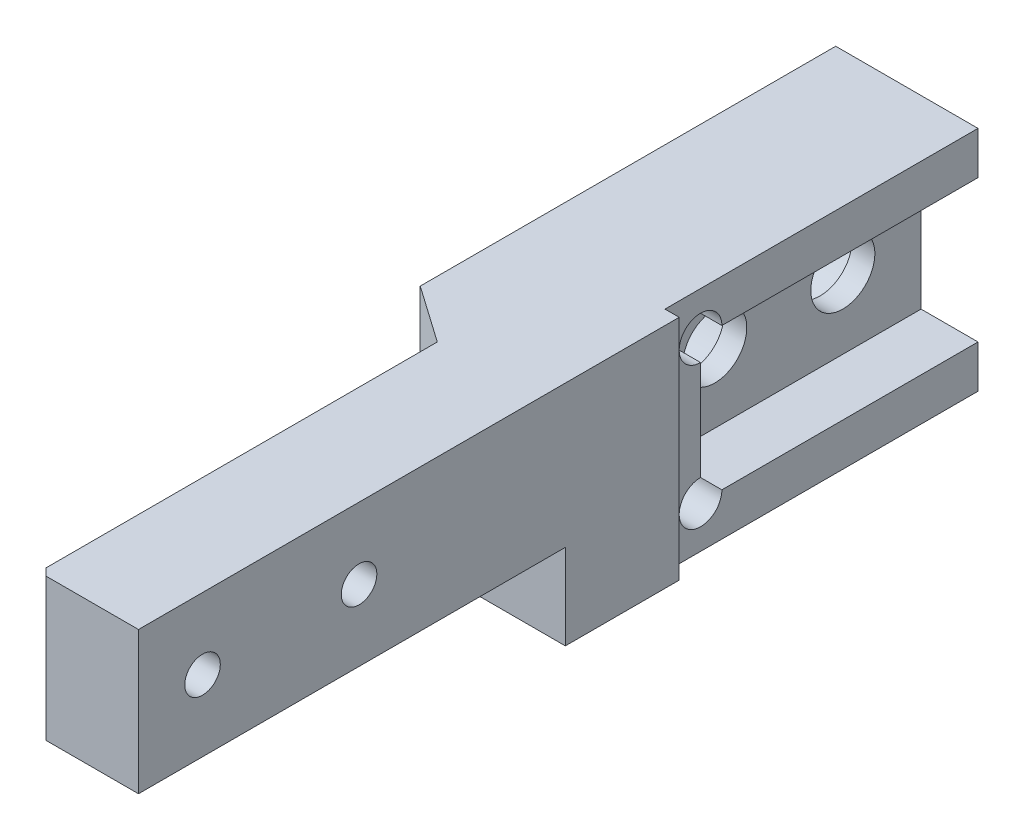
SolidWorks part; units mm, degrees
material "AL6061"
ref_plane "前视基准面" through (0, 0, 0) normal (0, 0, 1) x (1, 0, 0)
ref_plane "上视基准面" through (0, 0, 0) normal (0, 1, 0) x (1, 0, 0)
ref_plane "右视基准面" through (0, 0, 0) normal (1, 0, 0) x (0, 0, -1)
sketch "草图1" plane through (0, 0, 0) normal (0, 1, 0) x (1, 0, 0)
  line L1 (-10, 30) -> (10, 30)
  line L2 (-10, 30) -> (-10, -30)
  line L3 (-10, -30) -> (10, -30)
  line L4 (10, 30) -> (10, -30)
  line L5 (-10, 30) -> (10, -30) construction
  line L6 (-10, -30) -> (10, 30) construction
  point P0 (0, 0)
  dimension "D1" = 20
  dimension "D2" = 60
extrude "凸台-拉伸1" add sketch "草图1" along normal mid plane 16
sketch "草图2" plane through (10, 0, 0) normal (1, 0, 0) x (0, 0, -1)
  line L0 (0, 0) -> (45.4004, 0) construction
  line L1 (30, 8) -> (30, -8) construction
  line L2 (30, 5) -> (10.5, 5)
  line L3 (30, 5) -> (30, -5)
  line L4 (30, -5) -> (10.5, -5)
  line L5 (10.5, 5) -> (10.5, -5)
  dimension "D1" = 10
  dimension "D2" = 19.5
extrude "切除-拉伸1" cut sketch "草图2" against normal blind 14
sketch "草图3" [suppressed] plane through (0, -10, 0) normal (0, -1, 0) x (1, 0, 0)
  line L0 (13.3, -30) -> (13.3, 30) construction
  line L1 (13.3, 41.1716) -> (10, 43.5284)
  line L3 (13.3, 51.6213) -> (11, 49.3213)
  line L4 (12.5, -30) -> (-12.5, -30) construction
  line L5 (-12.5, 30) -> (12.5, 30) construction
  line L6 (12.5, 30) -> (12.5, -30) construction
  line L7 (13.3, -8.9282) -> (5.5, -4.4249)
  line L8 (13.3, -2) -> (7.3, -2) construction
  line L9 (13.3, 4.9282) -> (5.5, 0.4249)
  line L10 (5.5, 0.4249) -> (5.5, -4.4249)
  line L11 (13.3, 13) -> (8.3, 13) construction
  line L12 (13.3, 19.1039) -> (7.3, 14.9026)
  line L13 (13.3, 6.8961) -> (7.3, 11.0974)
  line L14 (7.3, 11.0974) -> (7.3, 14.9026)
  line L15 (13.3, 30.8831) -> (8, 27.172)
  line L16 (13.3, 26) -> (9.3, 26) construction
  line L17 (13.3, 21.1169) -> (8, 24.828)
  line L18 (8, 27.172) -> (8, 24.828)
  line L19 (13.3, 39.6623) -> (9, 36.6514)
  line L20 (13.3, 36) -> (10.3, 36) construction
  line L21 (9, 36.6514) -> (9, 35.3486)
  line L22 (13.3, 32.3377) -> (9, 35.3486)
  line L23 (13.3, 44) -> (11.3, 44) construction
  line L24 (13.3, 46.8284) -> (10, 43.5284)
  line L25 (13.3, 49.5) -> (11.8, 49.5) construction
  line L26 (13.3, 47.3787) -> (11, 49.3213)
  line L28 (13.3, 51.6213) -> (13.3, 47.3787)
  line L29 (13.3, 46.8284) -> (13.3, 41.1716)
  line L30 (13.3, 39.6623) -> (13.3, 32.3377)
  line L31 (13.3, 30.8831) -> (13.3, 21.1169)
  line L32 (13.3, 19.1039) -> (13.3, 6.8961)
  line L33 (13.3, 4.9282) -> (13.3, -8.9282)
  circle A0 centre (13.3, 49.5) radius 1.5 construction
  circle A1 centre (13.3, 44) radius 2 construction
  circle A2 centre (13.3, 36) radius 3 construction
  circle A3 centre (13.3, 26) radius 4 construction
  circle A4 centre (13.3, 13) radius 5 construction
  circle A5 centre (13.3, -2) radius 6 construction
  dimension "D2" = 3
  dimension "D3" = 4
  dimension "D4" = 6
  dimension "D5" = 8
  dimension "D6" = 10
  dimension "D7" = 12
  dimension "D8" = 2
  dimension "D9" = 3
  dimension "D10" = 3
  dimension "D11" = 4
  dimension "D12" = 4
  dimension "D13" = 0.8
  dimension "D14" = 28
  dimension "D15" = 30
  dimension "D16" = 7
  dimension "D17" = 35
  dimension "D18" = 6
  dimension "D19" = 35
  dimension "D20" = 4.5
  dimension "D21" = 35
  dimension "D22" = 3.5
  dimension "D23" = 45
  dimension "D24" = 2.5
  dimension "D25" = 45
  dimension "D26" = 1.5
sketch "草图4" plane through (0, -8, 0) normal (0, -1, 0) x (1, 0, 0)
  line L0 (11, 31.4426) -> (11, -30.9478) construction
  line L1 (10, 30) -> (10, -30) construction
  line L2 (10, 28.0377) -> (0.4211, 20)
  line L3 (-10, 30) -> (10, 30) construction
  line L4 (11, 20) -> (-10.1578, 20) construction
  line L5 (10, 11.9623) -> (0.4211, 20)
  line L6 (10, 28.0377) -> (10, 11.9623)
  line L7 (-10, -30) -> (-10, 30) construction
  circle A0 centre (11, 20) radius 6.8 construction
  dimension "D2" = 13.6
  dimension "D1" = 1
  dimension "D3" = 10
  dimension "D4" = 40
  dimension "D5" = 21
extrude "切除-拉伸2" [suppressed] cut sketch "草图4" against normal through all
fillet "圆角1" [suppressed] radius 2
chamfer "倒角1" distance 3 angle 45 2 edges at (10, 6.5, -30) (10, -6.5, -30)
sketch "草图5" plane through (0, -8, 0) normal (0, -1, 0) x (1, 0, 0)
  line L0 (-6, 30) -> (-6, 2)
  line L1 (-10, 30) -> (10, 30) construction
  line L2 (-6, 2) -> (-10, -0.8008)
  line L3 (-10, -30) -> (-10, 30) construction
  line L4 (10, 30) -> (10, -27) construction
  dimension "D1" = 16
  dimension "D2" = 125
  dimension "D3" = 28
extrude "切除-拉伸3" cut sketch "草图5" against normal through all and the other way through all flip side to cut
chamfer "倒角2" distance 0.5 angle 45 2 edges at (10, 0, 30) (-6, 0, 30)
sketch "草图6" plane through (10, 0, 0) normal (1, 0, 0) x (0, 0, -1)
  circle A0 centre (10.5, 5) radius 1.5
  circle A1 centre (10.5, -5) radius 1.5
  dimension "D1" = 3
extrude "切除-拉伸4" cut sketch "草图6" against normal up to surface (14 mm away) up to face at (-4, 0, -20.25)
sketch "草图7" plane through (-10, 0, 0) normal (-1, 0, 0) x (0, 0, 1)
  point P0 (-15.5, 0)
  point P3 (-24.5, 0)
hole_wizard "M4 六角凹头螺钉的柱形沉头孔1" positions "草图7" profile "草图8" counterbore size "M4" standard "ISO" end condition through all
sketch "草图8" plane through (-10, 0, -15.5) normal (0, 1, 0) x (0, 0, 1)
  line L0 (0, 0) -> (0, 20)
  line L1 (0, 20) -> (2.25, 20)
  line L3 (2.25, 20) -> (2.25, 4.4)
  line L4 (2.25, 4.4) -> (4, 4.4)
  line L5 (4, 4.4) -> (4, 0)
  line L7 (4, 0) -> (0, 0)
  line L11 (0, -6.35) -> (0, 107.95) construction
  dimension "通孔孔直径" = 4.5
  dimension "通孔孔深度" = 20
  dimension "柱形沉头孔直径" = 8
  dimension "柱形沉头孔深度" = 4.4
sketch "草图11" plane through (0, -8, 0) normal (0, -1, 0) x (1, 0, 0)
  line L0 (7, -30) -> (-10, -30) construction
  line L1 (0, -30) -> (10, -30)
  line L2 (0, -30) -> (0, -8)
  line L3 (0, -8) -> (10, -8)
  line L4 (10, -30) -> (10, -8)
  line L5 (10, 29.5) -> (10, -27) construction
  line L6 (-10, -30) -> (-10, -0.8008) construction
  dimension "D1" = 10
  dimension "D2" = 22
extrude "切除-拉伸7" cut sketch "草图11" against normal through all
sketch "草图12" plane through (10, 0, 0) normal (1, 0, 0) x (0, 0, -1)
  line L0 (-30, -8) -> (-30, 8) construction
  line L1 (-30, -8) -> (0, -8)
  line L2 (-30, -8) -> (-30, -2)
  line L3 (-30, -2) -> (0, -2)
  line L4 (0, -8) -> (0, -2)
  line L5 (-29.5, -8) -> (8, -8) construction
  line L7 (-29.5, 8) -> (8, 8) construction
  dimension "D1" = 10
  dimension "D2" = 30
extrude "切除-拉伸8" cut sketch "草图12" against normal through all
sketch "草图13" plane through (0, -2, 0) normal (0, -1, 0) x (1, 0, 0)
  line L1 (10, 14.2142) -> (5.9487, 20)
  line L2 (10, 0) -> (10, 29.5) construction
  line L3 (-5.5, 30) -> (9.5, 30) construction
  line L4 (14.25, 20) -> (-2.0615, 20) construction
  line L5 (10, 25.7858) -> (5.9487, 20)
  line L6 (10, 14.2142) -> (10, 25.7858)
  circle A0 centre (14.25, 20) radius 6.8 construction
  dimension "D1" = 13.6
  dimension "D2" = 4.25
  dimension "D3" = 10
  dimension "D4" = 110
extrude "切除-拉伸9" cut sketch "草图13" against normal through all
fillet "圆角2" radius 3 1 edges at (5.9487, 3, 20)
sketch "草图14" plane through (0, 8, 0) normal (0, 1, 0) x (1, 0, 0)
  line L0 (-6, -29.5) -> (-6, -2) construction
  line L1 (1, 15.4497) -> (19.5116, 15.4497)
  line L2 (1, 15.4497) -> (1, -40.8339)
  line L3 (1, -40.8339) -> (19.5116, -40.8339)
  line L4 (19.5116, 15.4497) -> (19.5116, -40.8339)
  dimension "D1" = 7
extrude "切除-拉伸10" cut sketch "草图14" against normal through all
hole_wizard "M3 螺纹孔1" positions "草图15" profile "草图16" tap size "M3" standard "GB" end condition through all
sketch "草图15" plane through (1, 0, 0) normal (1, 0, 0) x (0, 0, -1)
  line L0 (-30, 3) -> (-25.5, 3) construction
  line L1 (-30, -2) -> (-30, 8) construction
  point P0 (-25.5, 3)
  point P2 (-14.5, 3)
  dimension "D1" = 11
  dimension "D2" = 4.5
sketch "草图16" plane through (1, 3, 25.5) normal (0, 1, 0) x (0, 0, -1)
  line L0 (0, 0) -> (0, 11)
  line L1 (0, 11) -> (1.25, 11)
  line L2 (1.25, 11) -> (1.25, 0)
  line L5 (1.25, 0) -> (0, 0)
  line L11 (0, -6.35) -> (0, 107.95) construction
  dimension "通孔螺纹孔钻头直径" = 2.5
  dimension "通孔螺纹孔钻头深度" = 11
cosmetic thread "孔螺蚊线1" parameters "D2"=3
cosmetic thread "孔螺蚊线2" parameters "D2"=3
